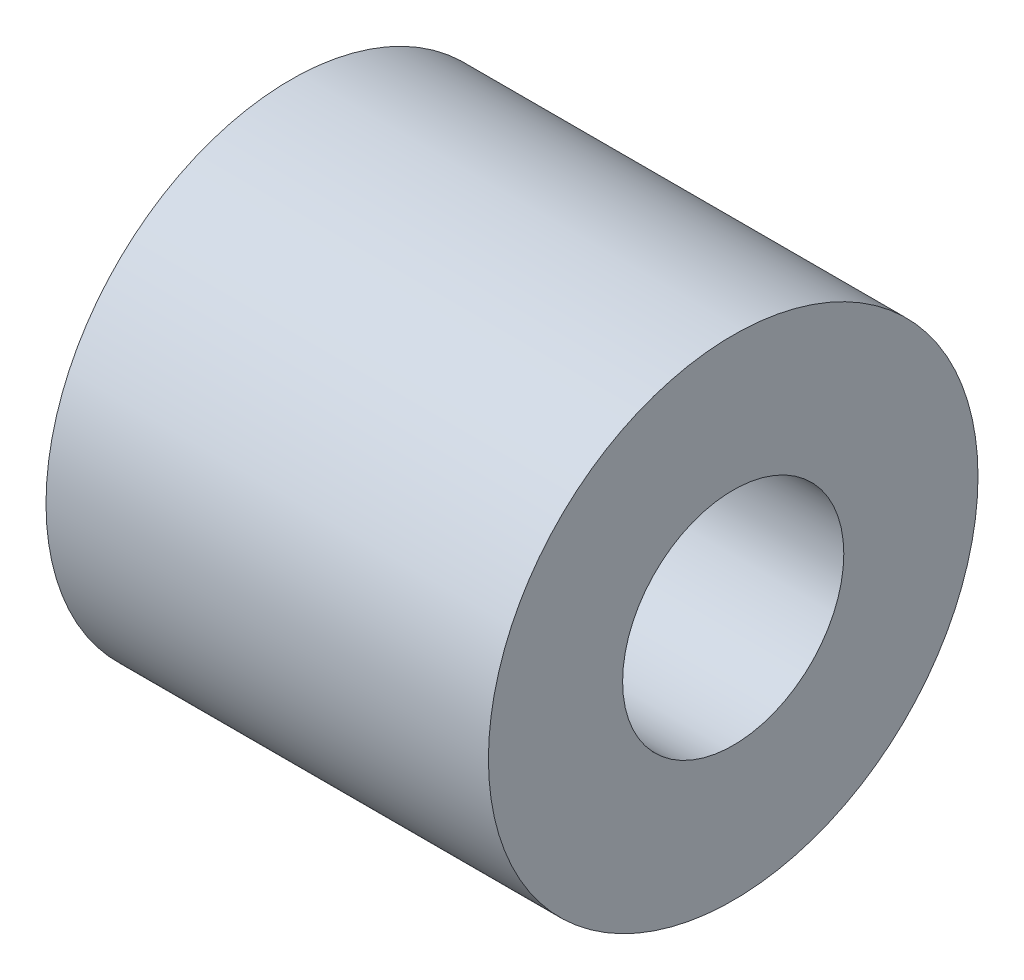
SolidWorks part; units mm, degrees
ref_plane "Front Plane" through (0, 0, 0) normal (0, 0, 1) x (1, 0, 0)
ref_plane "Top Plane" through (0, 0, 0) normal (0, 1, 0) x (1, 0, 0)
ref_plane "Right Plane" through (0, 0, 0) normal (1, 0, 0) x (0, 0, -1)
other "Configuration Table"
sketch "Sketch1" plane through (0, 0, 0) normal (1, 0, 0) x (0, 0, -1)
  circle A0 centre (0, 0) radius 375
  circle A1 centre (0, 0) radius 830
  dimension "D1" = 750
  dimension "D2" = 1660
extrude "Boss-Extrude1" add sketch "Sketch1" along normal blind 1500
